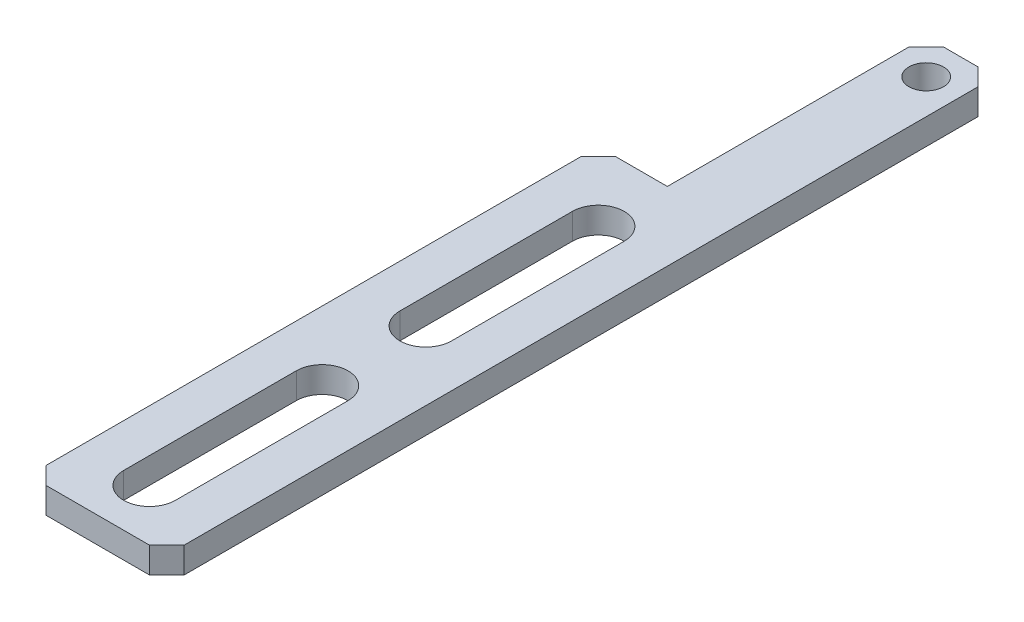
from build123d import *

# Parameters (mm, degrees)
SKETCH1_W                      = 8
SKETCH1_H                      = 48
BOSS_EXTRUDE1_DEPTH            = 1.5
F_2_5_2_5_DIAMETER_HOLE1_D     = 2
F_2_5_2_5_DIAMETER_HOLE1_DEPTH = 5
F_2_5_2_5_DIAMETER_HOLE1_TIP   = 0.600860619
SKETCH6_W                      = 4
SKETCH6_H                      = 15
CUT_EXTRUDE1_DEPTH             = 10
SKETCH7_R                      = 1.5
CUT_EXTRUDE2_DEPTH             = 10
CHAMFER1_SIZE                  = 1
CUT_EXTRUDE3_DEPTH             = 10


with BuildPart() as part:
    # Sketch1 → Boss-Extrude1 (new body)
    with BuildSketch(Plane(origin=(0, 0, 0), x_dir=(1, 0, 0), z_dir=(0, 1, 0))):
        with Locations((4, 24)):
            Rectangle(SKETCH1_W, SKETCH1_H)
    extrude(amount=BOSS_EXTRUDE1_DEPTH)

    # Ø2.5 (2.5) Diameter Hole1
    with Locations(Plane(origin=(0, 1.5, 0), x_dir=(1, 0, 0), z_dir=(0, 1, 0))):
        with Locations((6, 46)):
            Hole(F_2_5_2_5_DIAMETER_HOLE1_D / 2, depth=F_2_5_2_5_DIAMETER_HOLE1_DEPTH)
            with Locations((0, 0, -(F_2_5_2_5_DIAMETER_HOLE1_DEPTH + F_2_5_2_5_DIAMETER_HOLE1_TIP / 2))):  # 118° drill point
                Cone(0, F_2_5_2_5_DIAMETER_HOLE1_D / 2, F_2_5_2_5_DIAMETER_HOLE1_TIP, mode=Mode.SUBTRACT)

    # Sketch6 → Cut-Extrude1 (cut)
    with BuildSketch(Plane(origin=(0, 1.5, 0), x_dir=(1, 0, 0), z_dir=(0, 1, 0))):
        with Locations((2, 40.5)):
            Rectangle(SKETCH6_W, SKETCH6_H)
    extrude(amount=-CUT_EXTRUDE1_DEPTH, mode=Mode.SUBTRACT)

    # Sketch7 → Cut-Extrude2 (cut)
    with BuildSketch(Plane(origin=(0, 1.5, 0), x_dir=(1, 0, 0), z_dir=(0, 1, 0))):
        with Locations(Location((4, 24, 0), (0, 0, 270))):
            Circle(SKETCH7_R)
        with Locations(Location((4, 8, 0), (0, 0, 270))):
            Circle(SKETCH7_R)
    extrude(amount=-CUT_EXTRUDE2_DEPTH, mode=Mode.SUBTRACT)

    # Chamfer1
    chamfer1_edges = [part.edges().sort_by_distance(p)[0] for p in [
        (0, 0.75, -33),
        (4, 0.75, -48),
        (8, 0.75, -48),
        (8, 0.75, 0),
        (0, 0.75, 0),
    ]]
    chamfer(chamfer1_edges, length=CHAMFER1_SIZE)

    # Sketch8 → Cut-Extrude3 (cut)
    with BuildSketch(Plane(origin=(0, 1.5, 0), x_dir=(1, 0, 0), z_dir=(0, 1, 0))):
        with BuildLine():
            Line((5.5, 29), (5.5, 19))
            ThreePointArc((5.5, 19), (4, 17.5), (2.5, 19))
            Line((2.5, 19), (2.5, 29))
            ThreePointArc((2.5, 29), (4, 30.5), (5.5, 29))
        make_face()
        with BuildLine():
            Line((2.5, 3), (2.5, 13))
            ThreePointArc((2.5, 13), (4, 14.5), (5.5, 13))
            Line((5.5, 13), (5.5, 3))
            ThreePointArc((5.5, 3), (4, 1.5), (2.5, 3))
        make_face()
    extrude(amount=-CUT_EXTRUDE3_DEPTH, mode=Mode.SUBTRACT)


solid = part.part
